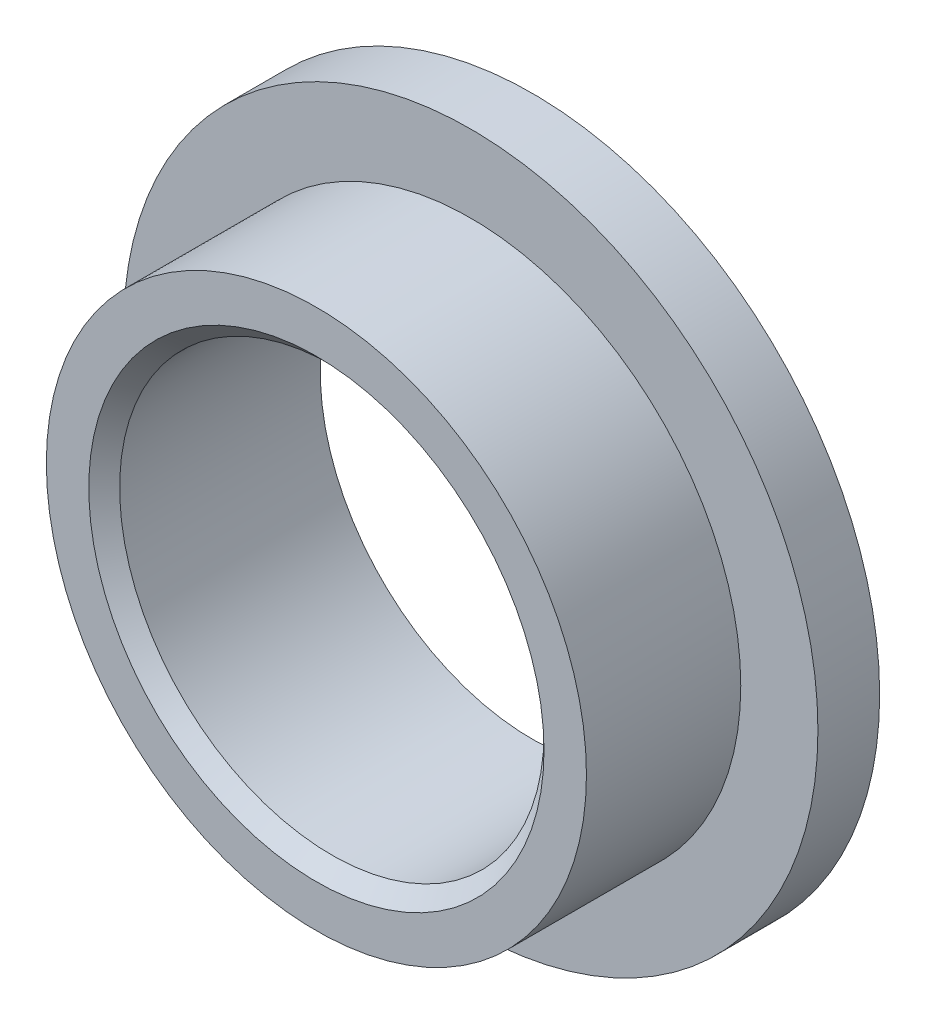
SolidWorks part; units mm, degrees
ref_plane "Front Plane" through (0, 0, 0) normal (0, 0, 1) x (1, 0, 0)
ref_plane "Top Plane" through (0, 0, 0) normal (0, 1, 0) x (1, 0, 0)
ref_plane "Right Plane" through (0, 0, 0) normal (1, 0, 0) x (0, 0, -1)
sketch "Sketch1" plane through (0, 0, 0) normal (0, 0, 1) x (1, 0, 0)
  circle A0 centre (0, 0) radius 27.5
  circle A1 centre (0, 0) radius 45
  dimension "D1" = 55
  dimension "D2" = 90
extrude "Boss-Extrude1" add sketch "Sketch1" along normal blind 28
sketch "Sketch2" plane through (0, 0, 28) normal (0, 0, 1) x (1, 0, 0)
  circle A0 centre (0, 0) radius 35
  circle A1 centre (0, 0) radius 45 construction
  circle A2 centre (0, 0) radius 45
  dimension "D1" = 70
extrude "Cut-Extrude1" cut sketch "Sketch2" against normal blind 20
chamfer "Chamfer1" distance 2 angle 45 1 edges at (27.5, 0, 28)
